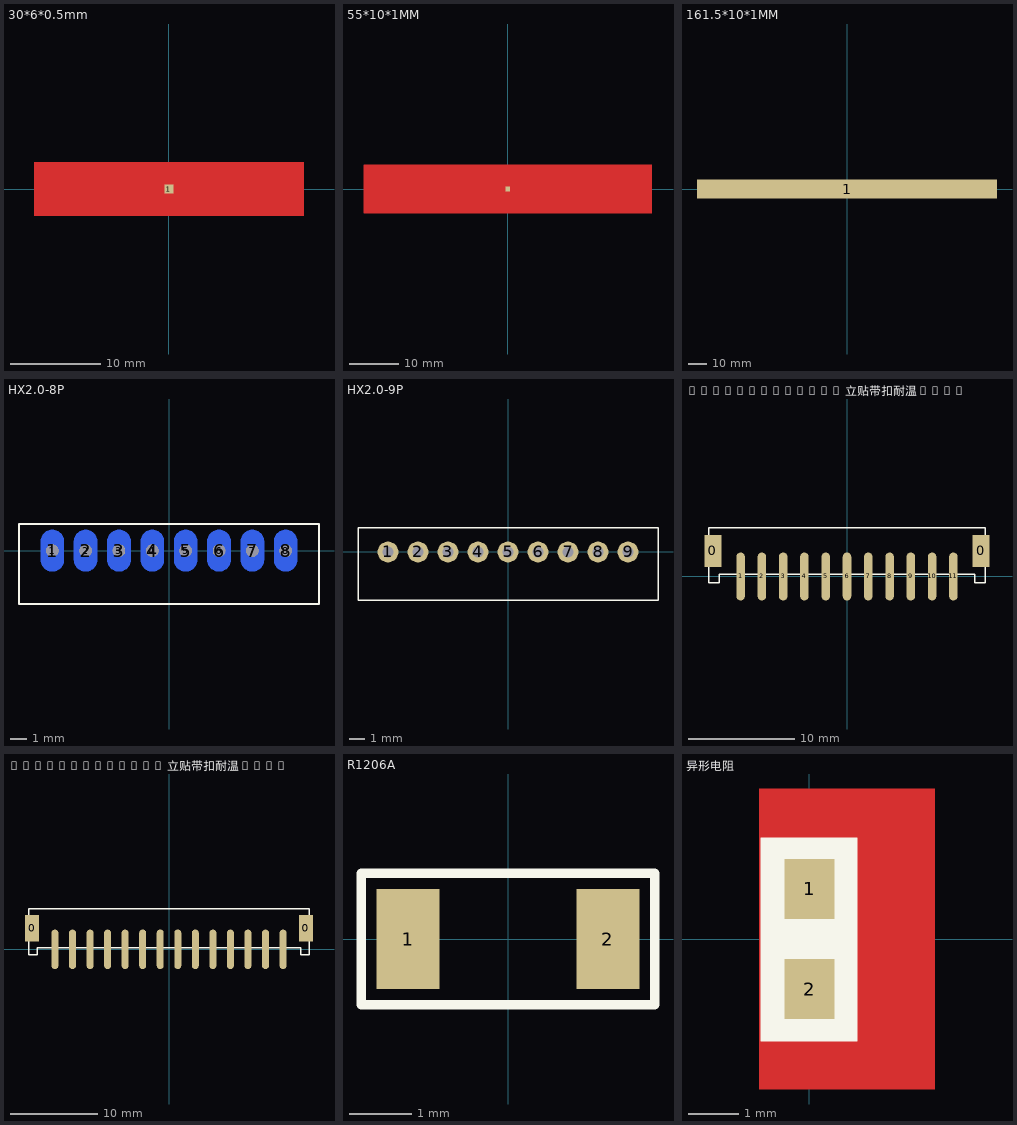
[diagram p0: the footprints below, top view; thin cyan lines are the x and y axes]
# Altium footprint library MISC86336.PcbLib: 9 footprints
Each footprint in its own frame and in the unit in brackets; x right, y up, seen from the top. Pads: shape width x height; smd on the part's side, far side on the other; paste and mask are expansions set on the pad; w line width, h text height; cw(c..) or ccw(c..) is an arc to the next point about the centre after c.

## 30*6*0.5mm [mm]
height 0.5
pads (1):
  rect 1x1 smd: 1(0,0)
Top Layer:
  rectangle: -14.999,-3 15.001,3
Top Solder:
  rectangle: -14.9,1.15 14.95,2.95
  rectangle: -14.95,-2.95 14.95,-1.15
  region: -14.95,2.95 -14.95,-2.95 -12.47,-2.95 -12.47,2.95
  region: -1.1,2.951 -1.1,-2.949 1.1,-2.949 1.1,2.951
  region: 12.518,2.95 12.518,-2.95 14.948,-2.95 14.948,2.95

## 55*10*1MM [mm]
pads (1):
  rect 1x1 smd: 1(0,0)
Top Layer:
  rectangle: -29.499,-5 29.501,5
Top Solder:
  region: 24.049,4.919 24.049,-4.982 27.479,-4.982 27.479,4.919
  rectangle: -27.4,2.15 27.45,4.95
  rectangle: -27.45,-4.95 27.45,-2.15
  region: -27.45,4.887 -27.45,-4.95 -23.97,-4.95 -23.97,4.887
  region: -2.1,4.9 -2.1,-4.949 2.1,-4.949 2.1,4.9

## 161.5*10*1MM [mm]
pads (1):
  rect 161.5x10 smd: 1(0,0)

## HX2.0-8P [mm]
pads (16):
  oval 1.4x2.5 smd far side: 1(-7,0) 2(-5,0) 3(-3,0) 4(-1,0) 5(1,0) 6(3,0) 7(5,0) 8(7,0)
  round 0.75 hole 0.75: 1(-7,0) 2(-5,0) 3(-3,0) 4(-1,0) 5(1,0) 6(3,0) 7(5,0) 8(7,0)
Top Overlay:
  lines w0.1: -9,-3.2 9,-3.2 9,1.6 -9,1.6 -9,-3.2
Keep-Out Layer:
  drawing of 8 lines, arcs and shapes, not listed
Keep-Out Layer:
  circle w0.01: c-7,0 r0.375
  circle w0.01: c-5,0 r0.375
  circle w0.01: c-3,0 r0.375
  circle w0.01: c-1,0 r0.375
  circle w0.01: c7,0 r0.375
  circle w0.01: c5,0 r0.375
  circle w0.01: c3,0 r0.375
  circle w0.01: c1,0 r0.375

## HX2.0-9P [mm]
pads (9):
  round 1.4 hole 0.75: 1(-8,0) 2(-6,0) 3(-4,0) 4(-2,0) 5(0,0) 6(2,0) 7(4,0) 8(6,0) 9(8,0)
Top Overlay:
  lines w0.1: -10,-3.2 -10,1.6 10,1.6 10,-3.2 -10,-3.2

## HY2.0WT-11A/P 立贴带扣耐温260℃ [mm] "Vertical SMD connector"
pads (13):
  rect 1.6x3 smd: 0(-12.6,2.4) 0(12.6,2.4)
  oval 0.8x4.5 smd: 1(-10,0) 2(-8,0) 3(-6,0) 4(-4,0) 5(-2,0) 6(0,0) 7(2,0) 8(4,0) 9(6,0) 10(8,0) 11(10,0)
Top Overlay:
  lines w0.15: -13,-0.6 -12,-0.6 -12,0.2 12,0.2 12,-0.6 13,-0.6 13,4.6 -13,4.6 -13,-0.6

## HY2.0WT-14A/P 立贴带扣耐温260℃ [mm] "Vertical SMD connector"
pads (16):
  rect 1.6x3 smd: 0(-15.6,2.4) 0(15.6,2.4)
  oval 0.8x4.5 smd: 1(-13,0) 2(-11,0) 3(-9,0) 4(-7,0) 5(-5,0) 6(-3,0) 7(-1,0) 8(1,0) 9(3,0) 10(5,0) 11(7,0) 12(9,0) 13(11,0) 14(13,0)
Top Overlay:
  lines w0.15: -16,-0.6 -15,-0.6 -15,0.2 15,0.2 15,-0.6 16,-0.6 16,4.6 -16,4.6 -16,-0.6

## R1206A [mm] "SMD resistor"
height 0.5
pads (2):
  rect 1x1.6 smd: 1(-1.6,0) 2(1.6,0)
Top Overlay:
  lines w0.15: -2.35,-1.05 -2.35,1.05 2.35,1.05 2.35,-1.05 -2.35,-1.05

## 异形电阻 [mm]
pads (2):
  rect 1x1.2 smd mask+0: 1(0,1) 2(0,-1)
Top Layer:
  region: 0.5,0.125 0.5,2.55 0.5,2.575 0.481,2.621 0.446,2.656 0.4,2.675 0.375,2.675 -0.425,2.675 -0.44,2.675 -0.467,2.664 -0.489,2.642 -0.5,2.615 -0.5,2.6 -0.5,0.125
  region: -0.5,-2.625 -0.5,-2.635 -0.492,-2.653 -0.478,-2.667 -0.46,-2.675 -0.45,-2.675 0.4,-2.675 0.42,-2.675 0.457,-2.66 0.485,-2.632 0.5,-2.595 0.5,-2.575 0.5,-0.125 -0.5,-0.125
  pour cut-out: -1,3 2.5,3 2.5,-3 -1,-3
  lines w0.2: -0.325,2.5 0,2.5
  lines w0.35: -0.325,-2.5 1.525,-2.5 ccw(c1.525,-2) 1.525,-1.5 ; -0.325,2.5 1.525,2.5 cw(c1.525,2) 1.525,1.5 ; 1.5,-1.5 cw(c1.5,-1) 1.5,-0.5 ; 1.5,0.5 cw(c1.5,1) 1.5,1.5 ; 1.525,-0.5 ccw(c1.525,0) 1.525,0.5
Top Overlay:
  pour cut-out: 0.955,2.026 -0.979,2.026 -0.979,-2.044 0.955,-2.044
  lines w0.127: -0.762,-0.508 -0.762,-1.778 0.762,-1.778 0.762,-0.508 ; -0.762,0.508 -0.762,1.778 0.762,1.778 0.762,0.508
Top Solder:
  region: 0.5,0.625 0,0.125 -0.5,0.625
  region: 0.5,-0.625 0,-0.125 -0.5,-0.625